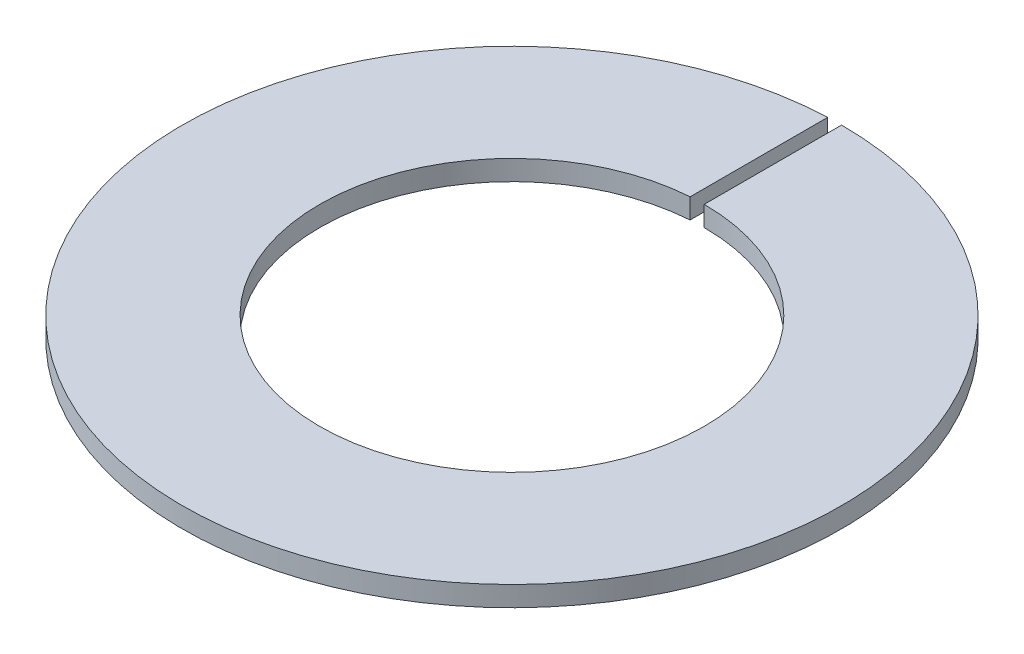
from build123d import *

# Parameters (mm, degrees)
BOSS_EXTRUDE1_DEPTH = 1.1


with BuildPart() as part:
    # Sketch1 → Boss-Extrude1 (new body)
    with BuildSketch(Plane(origin=(0, 0, 0), x_dir=(1, 0, 0), z_dir=(0, 1, 0))):
        with BuildLine():
            Line((0, 10.5), (0, 18))
            ThreePointArc((0, 18), (0.371526974, -17.996165361), (-0.742895651, 17.984663079))
            Line((-0.742895651, 17.984663079), (-0.742895651, 10.473686364))
            ThreePointArc((-0.742895651, 10.473686364), (0.371680762, -10.493419529), (0, 10.5))
        make_face()
    extrude(amount=BOSS_EXTRUDE1_DEPTH)


solid = part.part
